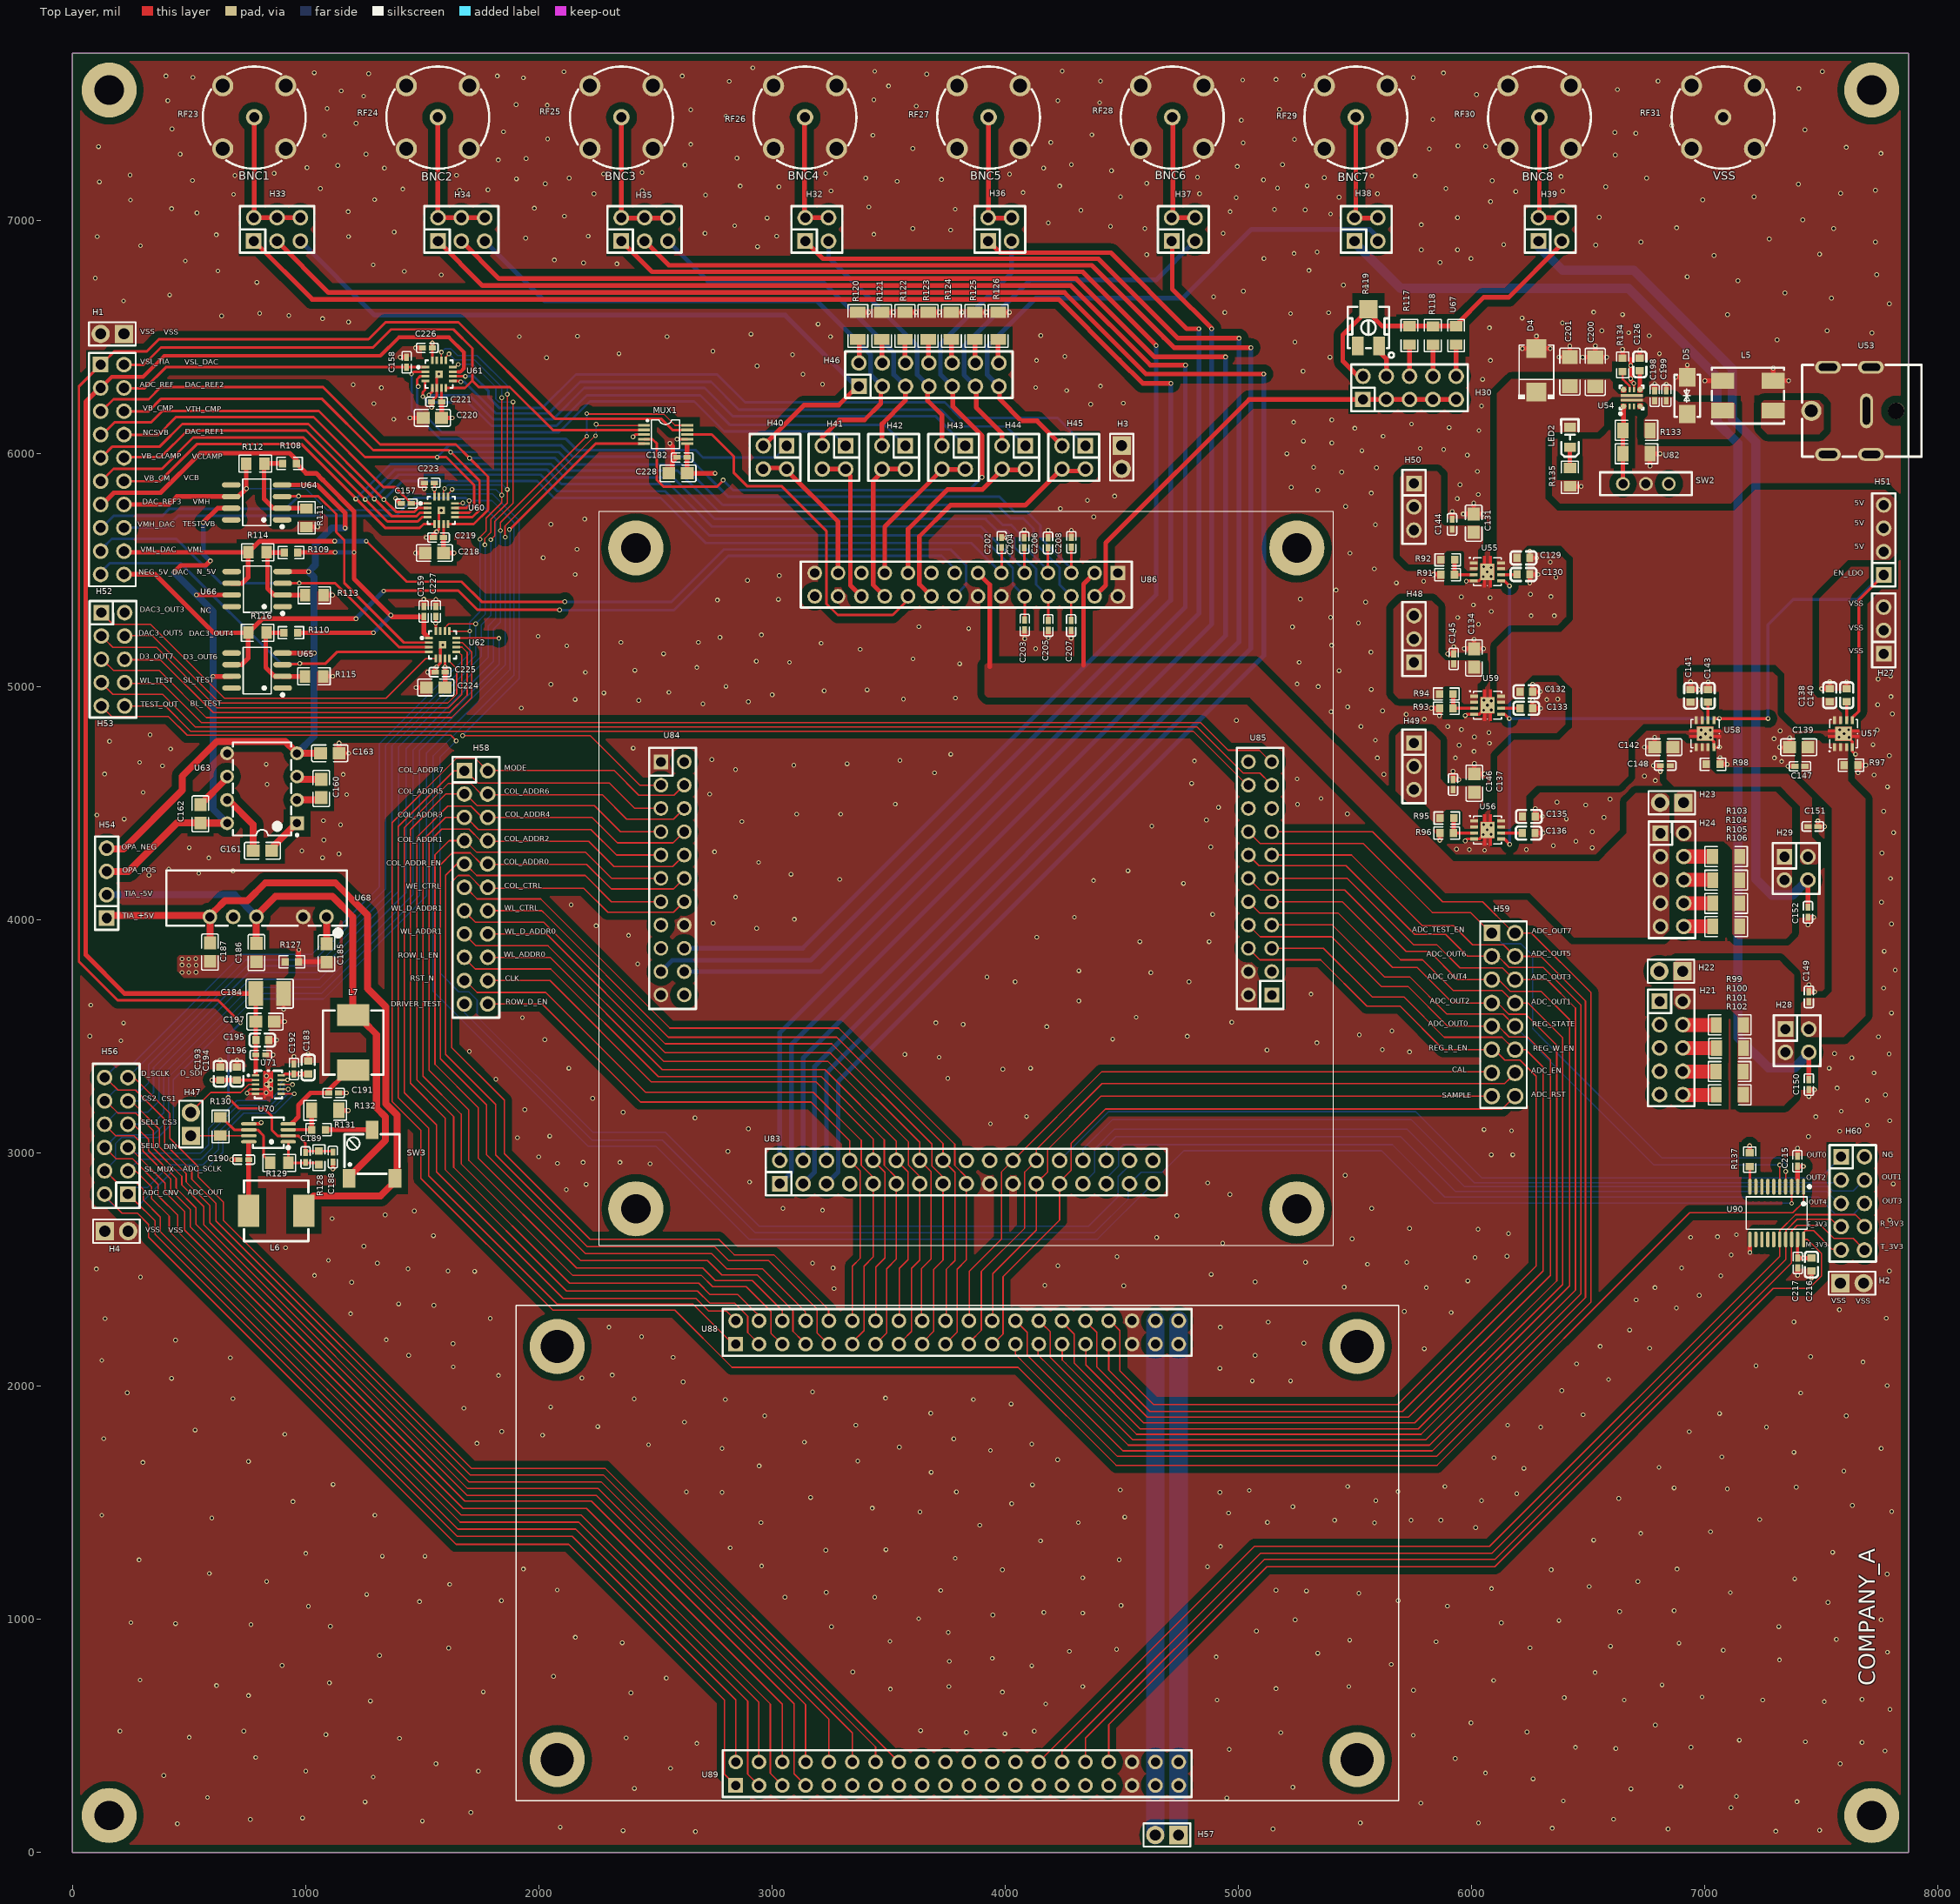
[diagram p0: Top Layer view]
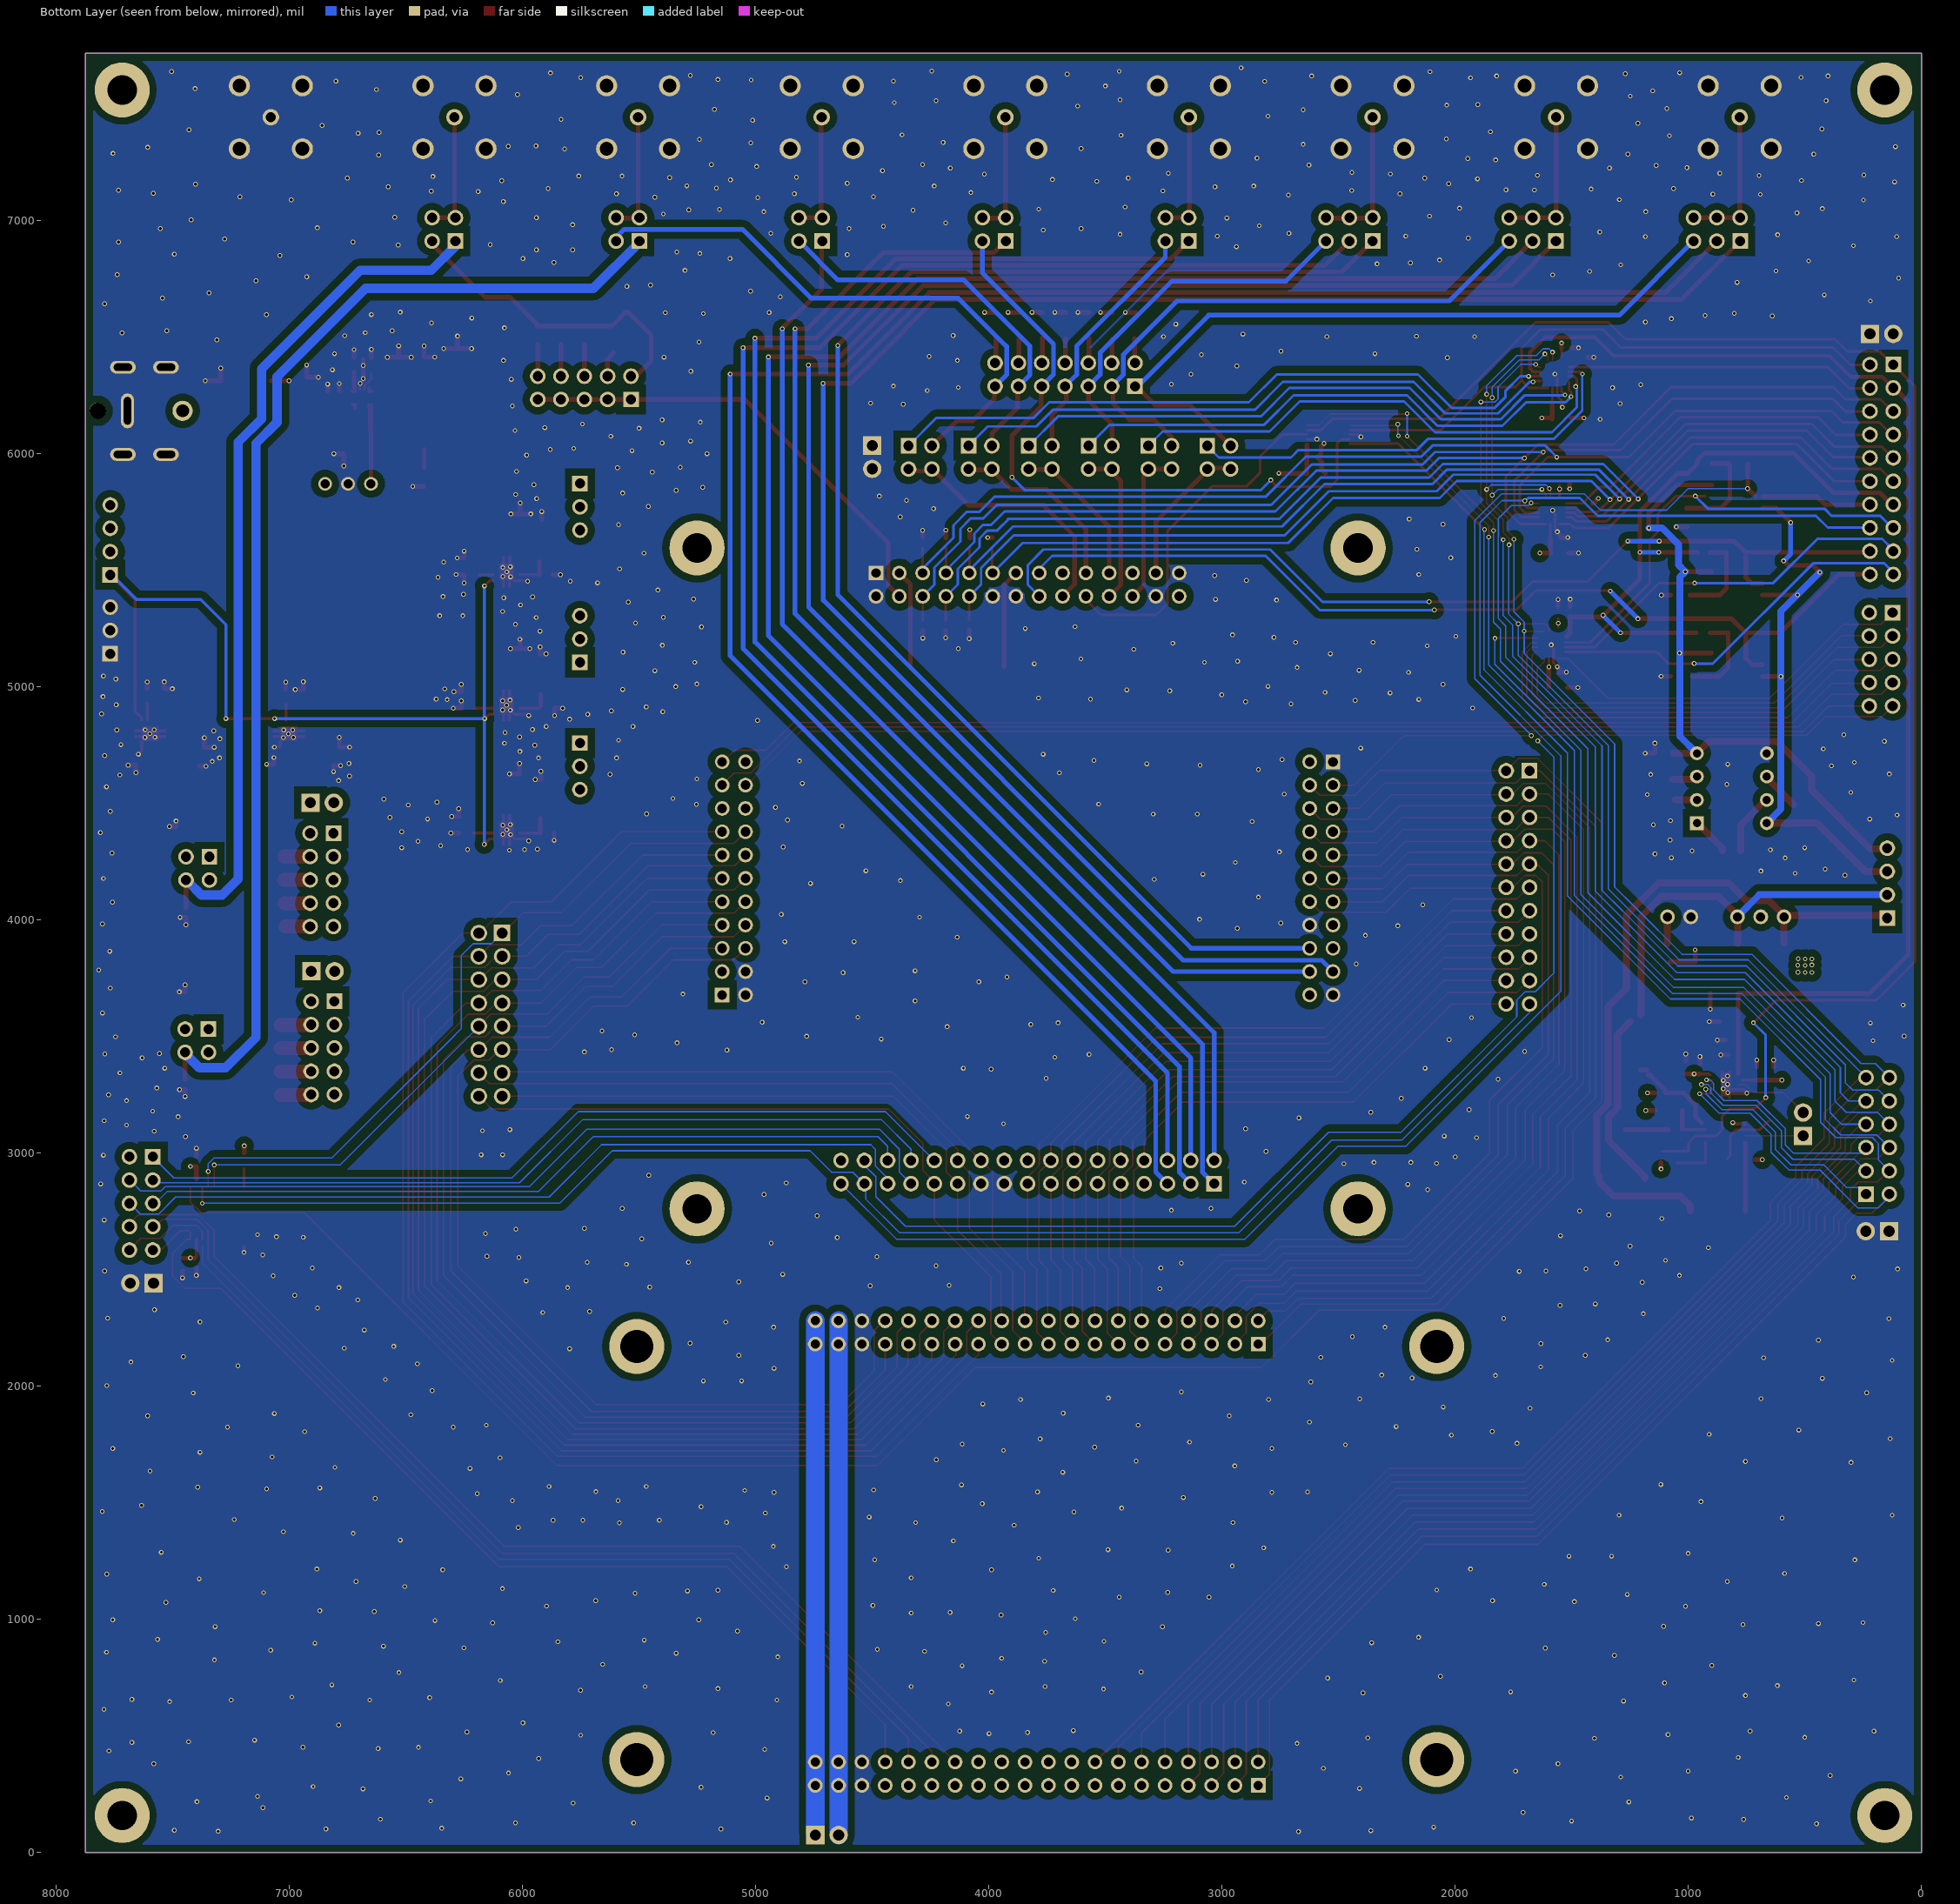
[diagram p1: Bottom Layer view, seen from below]
# Altium PCB MISC62793.pcbdoc (part 1 of 6)
Units mil, origin at the board's own origin, x right, y up, seen from the top; angles counter-clockwise.
Board outline 7874.02 x 7716.54 mil, 4 copper layers (Top Layer, GND, VCC, Bottom Layer); 201 components, 197 nets, 941 pads, 1215 vias.

## Layer stack, top to bottom (the 12.6 mil dielectric is the usual default, probably not edited)
Top Layer: signal copper 1.4
Dielectric: core 12.6, FR-4, Dk 4.8
GND: plane copper 1.4, net VSS
Dielectric: prepreg 12.6, FR-4, Dk 4.8
VCC: plane copper 1.4, net (Multiple Nets)
Dielectric: core 12.6, FR-4, Dk 4.8
Bottom Layer: signal copper 1.4

## Board outline
0,0 7874.02,0 7874.02,7716.54 0,7716.54

## Design rules (kind name [scope] priority, off if disabled: settings)
Clearance Clearance_1 [inpolygon] p1: gap=6
Clearance [All] p2: gap=6
DiffPairsRouting [All] p1: maxlimit=6 minlimit=6 mostfreqgap=6 maxuncoupledlength=500
HoleSize [All] p1: absolutevalues=TRUE maxlimit=500 minlimit=1 maxpercent=80.000 minpercent=20.000
HoleToHoleClearance [All] p1: gap=0 allowstackedmicrovias=TRUE
MinimumSolderMaskSliver [All] p1: minsoldermaskwidth=0
PlaneClearance [All] p1: clearance=6
PlaneConnect [All] p1: planeconnectstyle=Direct reliefexpansion=20 reliefentries=4 reliefconductorwidth=10 reliefairgap=10
PolygonConnect [All] p1: connectstyle=Direct reliefconductorwidth=10 reliefentries=4 polygonreliefangle="90 Angle"
RoutingVias [All] p1: holewidth=12 width=20 viastyle="Through Hole" minholewidth=12 minwidth=20 maxholewidth=12 maxwidth=20
SilkToSilkClearance [All] p1: silktosilkclearance=0
SilkscreenOverComponentPads SilkToSolderMaskClearance [IsPad] p1: minsilkscreentomaskgap=0
SolderMaskExpansion [All] p1: expansion=4
Width [All] p1: maxlimit=120 minlimit=6 preferedwidth=6 minimp=50.000000 maximp=50.000000 favimp=50.000000
20 further rules are at their usual default settings.

## Classes and differential pairs
component class 4_Digital.schdoc: C215 C216 C217 H57 H58 H59 H60 R137 U88 U89 U90
component class 3_ISC_Chip.schdoc: C202 C203 C204 C205 C206 C207 C208 U83 U84 U85 U86
component class 2_ADC_DAC.schdoc: C157 C158 C159 C160 C161 C162 C163 C182 C183 C184 C185 C186 C187 C188 C189 C190 C191 C192 C193 C194 C195 C196 C197 C218 C219 C220 C221 C223 C224 C225 C226 C227 C228 H30 H32 H33 H34 H35 H36 H37 H38 H39 H40 H41 H42 H43 H44 H45 H46 H47 H52 H53 H54 H56 L6 L7 MUX1 R108 R109 R110 R111 R112 R113 R114 R115 R116 R117 R118 R119 R120 R121 R122 R123 R124 R125 R126 R127 R128 R129 R130 R131 R132 RF23 RF24 RF25 RF26 RF27 RF28 RF29 RF30 RF31 SW3 U60 U61 U62 U63 U64 U65 U66 U67 U68 U70 U71
component class 1_Power.schdoc: C126 C129 C130 C131 C132 C133 C134 C135 C136 C137 C138 C139 C140 C141 C142 C143 C144 C145 C146 C147 C148 C149 C150 C151 C152 C198 C199 C200 C201 D4 D5 H1 H2 H3 H4 H21 H22 H23 H24 H27 H28 H29 H48 H49 H50 H51 L5 LED2 R91 R92 R93 R94 R95 R96 R97 R98 R99 R100 R101 R102 R103 R104 R105 R106 R133 R134 R135 SW2 U53 U54 U55 U56 U57 U58 U59 U82

## Components (designator, comment, footprint, x,y, rotation, side; value= is the part's Value field where it differs from the comment)
C126 "10nF" C0603 6722,6382 r270 top
C129 "1uF" C0603 6222.69,5551.85 r180 top
C130 "10nF" C0603 6222.69,5480.98 r180 top
C131 "4.7uF" C0805 6009.51,5700.99 r270 top
C132 "1uF" C0603 6234.93,4977.99 r180 top
C133 "10nF" C0603 6234.93,4906.99 r180 top
C134 "4.7uF" C0805 6010.93,5122.99 r270 top
C135 "1uF" C0603 6245.93,4442.99 r180 top
C136 "10nF" C0603 6244.93,4371.99 r180 top
C137 "4.7uF" C0805 6011.93,4585.99 r270 top
C138 "1uF" C0603 7536.65,4962.91 r270 top
C139 "4.7uF" C0805 7403.65,4739.91 r0 top
C140 "10nF" C0603 7609,4963 r270 top
C141 "1uF" C0603 6939.9,4960.18 r270 top
C142 "4.7uF" C0805 6824.9,4740.18 r0 top
C143 "10nF" C0603 7014.9,4960.18 r270 top
C144 "0.1uF" C0402 5917,5696 r270 top
C145 "0.1uF" C0402 5924,5119 r270 top
C146 "0.1uF" C0402 5921,4580 r270 top
C147 "0.1uF" C0402 7409,4658 r0 top
C148 "0.1uF" C0402 6831,4661 r0 top
C149 "0.1uF" C0402 7447,3669 r270 top
C150 "0.1uF" C0402 7447,3293 r90 top
C151 "0.1uF" C0402 7464,4400 r180 top
C152 "0.1uF" C0402 7443,4032 r90 top
C157 "150nF" C0402 1432.32,5785.23 r0 top
C158 "150nF" C0402 1433,6391 r270 top
C159 "150nF" C0402 1506.74,5322.01 r270 top
C160 "4.7uF" C0805 1067,4563 r270 top
C161 "4.7uF" C0805 815,4296 r0 top
C162 "4.7uF" C0805 549,4454 r270 top
C163 "4.7uF" C0805 1104,4714 r180 top
C182 "100nF" C0402 2615,5983 r0 top
C183 "1uF" C0603 1011,3366 r270 top
C184 "100uF" C1210 845.99,3683.05 r180 top
C185 "4.7uF" C0805 1090,3857 r270 top
C186 "4.7uF" C0805 789,3859 r270 top
C187 "4.7uF" C0805 590,3861 r270 top
C188 "68pF" C0402 1116.99,2982.05 r270 top
C189 "24pF" C0402 999.99,2980.05 r90 top
C190 "100nF" C0402 735,2971 r180 top
C191 "100nF" C0402 1120,3257 r180 top
C192 "100nF" C0402 950,3360 r90 top
C193 "1uF" C0603 633.99,3340.05 r90 top
C194 "1nF" C0603 705.99,3340.05 r90 top
C195 "1nF" C0603 813.99,3484.05 r180 top
C196 "100nF" C0402 807.99,3420.05 r0 top
C197 "10uF" C0805 825.99,3563.05 r180 top
C198 "100nF" C0402 6785.53,6247.99 r270 top
C199 "100nF" C0402 6835.53,6247.99 r270 top
C200 "22uF" C1206 6530.53,6349.99 r270 top
C201 "22uF" C1206 6422,6351 r270 top
C202 "100nF" C0402 3985,5618 r90 top
C203 "100nF" C0402 4084,5264 r270 top
C204 "100nF" C0402 4082,5617.46 r90 top
C205 "100nF" C0402 4185,5262 r270 top
C206 "100nF" C0402 4184,5616.46 r90 top
C207 "100nF" C0402 4283,5262 r270 top
C208 "100nF" C0402 4284,5618.46 r90 top
C215 "100nF" C0402 7398,2964 r270 top
C216 "1uF" C0603 7458,2521 r90 top
C217 "100nF" C0402 7399,2528 r90 top
C218 "10uF" C0805 1552.32,5573.23 r0 top
C219 "100nF" C0402 1570.32,5639.23 r0 top
C220 "10uF" C0805 1543.69,6152.44 r0 top
C221 "100nF" C0402 1561.69,6221.44 r0 top
C223 "100nF" C0402 1530,5874 r0 top
C224 "10uF" C0805 1558,4996 r0 top
C225 "100nF" C0402 1576.74,5062.01 r0 top
C226 "100nF" C0402 1522,6453 r0 top
C227 "100nF" C0402 1558.74,5322.01 r270 top
C228 "10uF" C0805 2597,5915 r0 top
D4 "#NAME?" SMB_L4.6-W3.6-LS5.3-RD 6278.53,6356.99 r90 top
D5 "#NAME?" SMA_L4.2-W2.7-LS5.0-BI 6925.53,6247.99 r270 top
H1 "#NAME?" HDR-TH_2P-P2.54-V-M 171,6513 r180 top
H2 "#NAME?" HDR-TH_2P-P2.54-V-M 7632,2441 r0 top
H3 "#NAME?" HDR-TH_2P-P2.54-V-M 4500,5984 r270 top
H4 "#NAME?" HDR-TH_2P-P2.54-V-M 189,2664 r0 top
H21 "#NAME?" HDR-TH_10P-P2.54-V-M-R2-C5-S2.54 6856.47,3450.01 r270 top
H22 "#NAME?" HDR-TH_2P-P2.54-V-M 6855.47,3779.01 r180 top
H23 "#NAME?" HDR-TH_2P-P2.54-V-M 6859,4502 r180 top
H24 "#NAME?" HDR-TH_10P-P2.54-V-M-R2-C5-S2.54 6860.47,4171.01 r270 top
H27 "#NAME?" HDR-TH_3P-P2.54-V-M 7768,5241 r90 top
H28 "#NAME?" HDR-TH_4P-P2.54-V-M-R2-C2-S2.54 7396.47,3481.01 r270 top
H29 "#NAME?" HDR-TH_4P-P2.54-V-M-R2-C2-S2.54 7392.47,4220.01 r270 top
H30 "#NAME?" HDR-TH_10P-P2.54-V-M-R2-C5-S2.54 5734.6,6281.6 r0 top
H32 "#NAME?" HDR-TH_4P-P2.54-V-M-R2-C2-S2.54 3192.61,6961 r0 top
H33 "#NAME?" HDR-TH_6P-P2.54-V-M-R2-C3-S2.54 877.64,6961 r0 top
H34 "#NAME?" HDR-TH_6P-P2.54-V-M-R2-C3-S2.54 1668,6961 r0 top
H35 "#NAME?" HDR-TH_6P-P2.54-V-M-R2-C3-S2.54 2453.8,6961 r0 top
H36 "#NAME?" HDR-TH_4P-P2.54-V-M-R2-C2-S2.54 3977.41,6961 r0 top
H37 "#NAME?" HDR-TH_4P-P2.54-V-M-R2-C2-S2.54 4764.21,6961 r0 top
H38 "#NAME?" HDR-TH_4P-P2.54-V-M-R2-C2-S2.54 5548.49,6961 r0 top
H39 "#NAME?" HDR-TH_4P-P2.54-V-M-R2-C2-S2.54 6337.61,6961 r0 top
H40 "#NAME?" HDR-TH_4P-P2.54-V-M-R2-C2-S2.54 3013,5983 r180 top
H41 "#NAME?" HDR-TH_4P-P2.54-V-M-R2-C2-S2.54 3266,5983 r180 top
H42 "#NAME?" HDR-TH_4P-P2.54-V-M-R2-C2-S2.54 3522,5983 r180 top
H43 "#NAME?" HDR-TH_4P-P2.54-V-M-R2-C2-S2.54 3779,5983 r180 top
H44 "#NAME?" HDR-TH_4P-P2.54-V-M-R2-C2-S2.54 4037,5983 r180 top
H45 "#NAME?" HDR-TH_4P-P2.54-V-M-R2-C2-S2.54 4294,5983 r180 top
H46 "#NAME?" HDR-TH_14P-P2.54-V-M-R2-C7-S2.54 3673,6338 r0 top
H47 "#NAME?" HDR-TH_2P-P2.54-V-M 508,3123 r90 top
H48 "#NAME?" HDR-TH_3P-P2.54-V-M 5753.73,5204 r90 top
H49 "#NAME?" HDR-TH_3P-P2.54-V-M 5753.73,4658 r270 top
H50 "#NAME?" HDR-TH_3P-P2.54-V-M 5753.31,5771 r270 top
H51 "#NAME?" HDR-TH_4P-P2.54-V-M 7768,5629 r90 top
H52 "#NAME?" HDR-TH_20P-P2.54-V-M-R2-C10-S2.54 171,5931 r270 top
H53 "#NAME?" HDR-TH_10P-P2.54-V-M-R2-C5-S2.54 174,5117 r270 top
H54 "#NAME?" HDR-TH_4P-P2.54-V-M 147,4157 r90 top
H56 "#NAME?" HDR-TH_12P-P2.54-V-M-R2-C6-S2.54 188,3073 r90 top
H57 "#NAME?" HDR-TH_2P-P2.54-V-M 4694,74 r180 top
H58 "#NAME?" HDR-TH_22P-P2.54-V-M-R2-C11-S2.54 1731,4139 r270 top
H59 "#NAME?" HDR-TH_16P-P2.54-V-M-R2-C8-S2.54 6137,3593 r270 top
H60 "#NAME?" HDR-TH_10P-P2.54-V-M-R2-C5-S2.54 7635.34,2783.46 r270 top
L5 "#NAME?" FILTER-SMD_4P-L7.0-W6.0-TL_SMCM7060 7185.53,6247.99 r180 top
L6 "10uH" IND-SMD_L7.3-W6.8 873.99,2751.05 r0 top
L7 "10uH" IND-SMD_L7.3-W6.8 1204,3473 r270 top
LED2 "LED_0805-R" LED_0805 6422.59,6071.01 r90 top
MUX1 "#NAME?" VSSOP-10_L3.0-W3.0-P0.50-LS4.9-BL 2544.01,6081.06 r270 top
R91 "10kΩ" R0603 5897.79,5479.67 r0 top
R92 "52.3kΩ" R0603 5898,5544 r180 top
R93 "10kΩ" R0603 5891.93,4906.99 r0 top
R94 "30.9kΩ" R0603 5891.93,4967.99 r0 top
R95 "12.5kΩ" R0603 5894.12,4436.21 r180 top
R96 "10kΩ" R0603 5893.93,4371.99 r0 top
R97 "10kΩ" R0603 7628,4663 r180 top
R98 "10kΩ" R0603 7036,4667 r180 top
R99 "1Ω" R1206 7107.47,3549.01 r0 top
R100 "10Ω" R1206 7108.47,3449.01 r0 top
R101 "100Ω" R1206 7107,3349 r0 top
R102 "100mΩ" R1206 7107.47,3249.01 r0 top
R103 "1Ω" R1206 7092,4271 r0 top
R104 "10Ω" R1206 7092.47,4170.01 r0 top
R105 "100Ω" R1206 7092.47,4070.01 r0 top
R106 "100mΩ" R1206 7092.47,3971.01 r0 top
R108 "10kΩ" R0603 931.39,5957.07 r180 top
R109 "10kΩ" R0603 937.39,5575.07 r180 top
R110 "10kΩ" R0603 937.12,5231.07 r180 top
R111 "20kΩ" R0805 1004.39,5724.07 r90 top
R112 "20kΩ" R0805 784.39,5956.07 r180 top
R113 "20kΩ" R0805 1037.39,5392.07 r180 top
R114 "20kΩ" R0805 794.39,5576.07 r180 top
R115 "20kΩ" R0805 1036.12,5044.07 r180 top
R116 "20kΩ" R0805 794.12,5231.07 r180 top
R117 "4kΩ" R0805 5734,6506 r90 top
R118 "5kΩ" R0805 5834.6,6505.6 r90 top
R119 "200kΩ" RES-ADJ-SMD_3P-L4.5-W4.5-P2.30-BL-FS 5558,6540 r90 top
R120 "1MΩ" R1206 3368.53,6546.99 r90 top
R121 "1MΩ" R1206 3470.53,6546.99 r90 top
R122 "1MΩ" R1206 3570.53,6546.99 r90 top
R123 "1MΩ" R1206 3669.53,6546.99 r90 top
R124 "1MΩ" R1206 3769.53,6546.99 r90 top
R125 "1MΩ" R1206 3870.53,6546.99 r90 top
R126 "1MΩ" R1206 3970,6547 r90 top
R127 "0Ω" R0603 941,3819 r0 top
R128 "10kΩ" R0603 1056.99,2979.05 r270 top
R129 "1kΩ" R0805 886.99,2957.05 r180 top
R130 "1kΩ" R0805 634.99,3113.05 r270 top
R131 "100kΩ" R0603 1056,3099 r180 top
R132 "100Ω" R1206 1084,3182 r180 top
R133 "1MΩ" R1206 6707.53,6098.99 r180 top
R134 "681Ω" R0603 6648,6380 r90 top
R135 "1kΩ" R0805 6422,5898 r90 top
R137 "10kΩ" R0603 7193,2971 r270 top
RF23 "#NAME?" ANT-TH_DOSIN-801-0057 779.64,7441.99 r0 top
RF24 "#NAME?" ANT-TH_DOSIN-801-0057 1567.04,7441.99 r0 top
RF25 "#NAME?" ANT-TH_DOSIN-801-0057 2354.45,7441.99 r0 top
RF26 "#NAME?" ANT-TH_DOSIN-801-0057 3141.85,7441.99 r0 top
RF27 "#NAME?" ANT-TH_DOSIN-801-0057 3929.25,7441.99 r0 top
RF28 "#NAME?" ANT-TH_DOSIN-801-0057 4716.65,7441.99 r0 top
RF29 "#NAME?" ANT-TH_DOSIN-801-0057 5504.05,7441.99 r0 top
RF30 "#NAME?" ANT-TH_DOSIN-801-0057 6291.45,7441.99 r0 top
RF31 "#NAME?" ANT-TH_DOSIN-801-0057 7078.86,7441.99 r0 top
SW2 "#NAME?" SW-TH_K3-1204D 6748,5870 r180 top
SW3 "50kΩ" RES-ADJ-SMD_3P-L6.0-W4.3-P5.00-BL 1285,2995 r0 top
U53 "#NAME?" DC-IN-TH_HX-DC007B-2.5 7585.53,6182.99 r180 top
U54 "#NAME?" VQFN-10_L2.0-W2.0-P0.45-TL 6687.53,6237.99 r90 top
U55 "#NAME?" VSON-8_L3.0-W3.0-P0.65-TL-EP 6068.08,5492.48 r0 top
U56 "#NAME?" VSON-8_L3.0-W3.0-P0.65-TL-EP 6068.93,4384.99 r0 top
U57 "#NAME?" VSON-8_L3.0-W3.0-P0.65-TL-EP 7595.65,4797.91 r90 top
U58 "#NAME?" VSON-8_L3.0-W3.0-P0.65-TL-EP 7001.9,4798.18 r90 top
U59 "#NAME?" VSON-8_L3.0-W3.0-P0.65-TL-EP 6068.93,4919.99 r0 top
U60 "#NAME?" WQFN-16_L3.0-W3.0-P0.50-TL-EP0.8 1582.12,5756.26 r0 top
U61 "#NAME?" WQFN-16_L3.0-W3.0-P0.50-TL-EP0.8 1572.69,6340.44 r0 top
U62 "#NAME?" WQFN-16_L3.0-W3.0-P0.50-TL-EP0.8 1587.74,5179.01 r0 top
U63 "#NAME?" DIP-8_L10.1-W6.3-P2.54-LS7.6-BL 813.39,4564.07 r90 top
U64 "#NAME?" SOIC-8_L4.9-W3.9-P1.27-LS6.0-BL 790.39,5790.07 r90 top
U65 "#NAME?" SOIC-8_L4.9-W3.9-P1.27-LS6.0-BL 792.17,5068.87 r90 top
U66 "#NAME?" SOIC-8_L4.9-W3.9-P1.27-LS6.0-BL 792.39,5418.07 r90 top
U67 "8kΩ" R0805 5934,6506 r90 top
U68 "#NAME?" PWRM-TH_A05XXS-1WR3 839.53,4012.48 r180 top
U70 "#NAME?" MSOP-8_L3.0-W3.0-P0.65-LS5.0-TL 840.99,3086.05 r180 top
U71 "#NAME?" VSON-10_L3.0-W3.0-P0.50-TL-EP-3 840.19,3293.02 r0 top
U82 "357kΩ" R1206 6707.53,5998.99 r0 top
U83 "#NAME?" HDR-TH_34P-P2.54-V-F-R2-C17-S2.54-1 3833.65,2917.62 r0 top
U84 "#NAME?" HDR-TH_22P-P2.54-V-F-R2-C11-S2.54 2573.81,4177.46 r270 top
U85 "#NAME?" HDR-TH_22P-P2.54-V-F-R2-C11-S2.54 5093.5,4177.46 r90 top
U86 "#NAME?" HDR-TH_28P-P2.54-V-F-R2-C14-S2.54-1 3833.65,5437.31 r180 top
U88 "#NAME?" HDR-TH_40P-P2.54-V-F-R2-C20-S2.54 3794.4,2229.91 r0 top
U89 "#NAME?" HDR-TH_40P-P2.54-V-F-R2-C20-S2.54 3794.4,337 r0 top
U90 "#NAME?" TSSOP-20_L6.5-W4.4-P0.65-LS6.4-BL 7309.14,2741.71 r180 top

## Footprints (in the part's own frame and the unit in brackets; to place one, negate y for a bottom-side part, rotate by r counter-clockwise, add the part's x,y. Pads: shape width x height; smd on the part's side, far side on the other; paste and mask are expansions set on the pad)
ANT-TH_DOSIN-801-0057 [mm]
  round 1.8 hole 1.1: 1(0,0)
  round 2.3 hole 1.5: 2(-3.429,3.429) 3(3.429,3.429) 4(3.429,-3.429) 5(-3.429,-3.429)
  silkscreen extent -5.6,-5.6 5.6,5.53